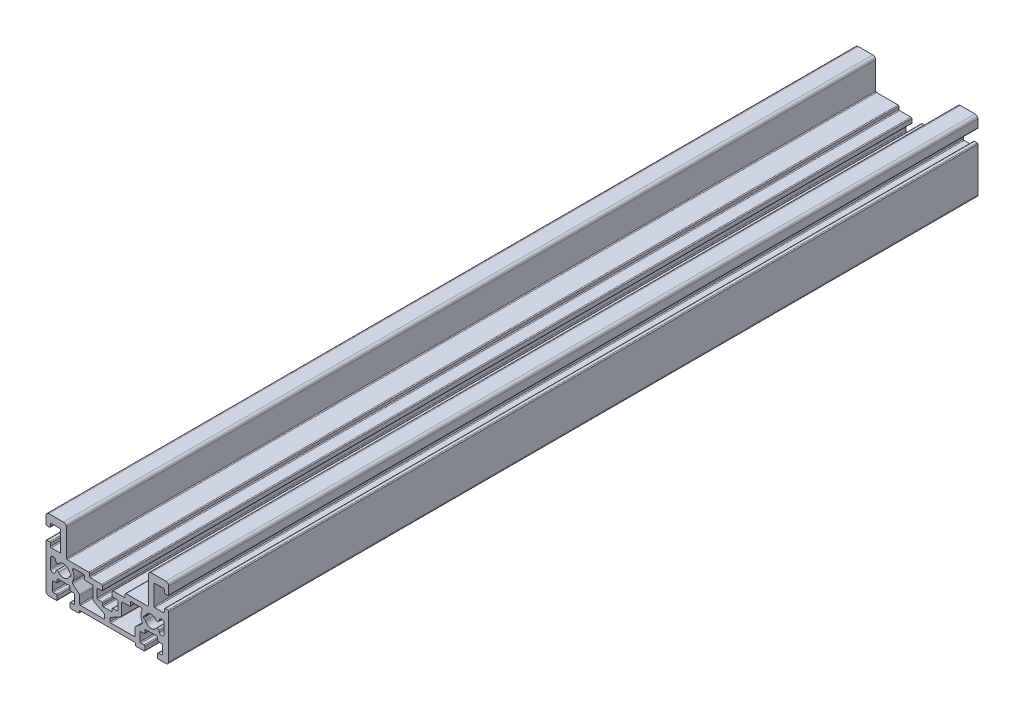
SolidWorks part; units mm, degrees
ref_plane "Front Plane" through (0, 0, 0) normal (0, 0, 1) x (1, 0, 0)
ref_plane "Top Plane" through (0, 0, 0) normal (0, 1, 0) x (1, 0, 0)
ref_plane "Right Plane" through (0, 0, 0) normal (1, 0, 0) x (0, 0, -1)
sketch "Sketch3" plane through (0, 0, 0) normal (0, 0, 1) x (1, 0, 0)
  line L214 (780.7533, -9071.888) -> (783.9435, -9071.888)
  line L215 (784.2435, -9072.188) -> (784.2435, -9073.188)
  line L216 (784.5435, -9073.488) -> (786.9435, -9073.488)
  line L217 (787.2435, -9073.788) -> (787.2435, -9077.8106)
  line L218 (787.399, -9078.0735) -> (791.0881, -9080.1025)
  line L219 (791.2435, -9080.3654) -> (791.2435, -9081.388)
  line L220 (790.9435, -9081.688) -> (782.9935, -9081.688)
  line L221 (782.6935, -9081.388) -> (782.6935, -9078.9167)
  line L222 (782.5205, -9078.5385) -> (780.2888, -9076.609)
  line L223 (772.6935, -9075.8786) -> (772.6935, -9072.6975)
  line L224 (779.4063, -9073.788) -> (779.3935, -9073.788)
  line L225 (779.6935, -9074.088) -> (779.6935, -9074.488)
  line L226 (779.3935, -9074.788) -> (779.4063, -9074.788)
  line L227 (803.9983, -9076.609) -> (801.7665, -9078.5385)
  line L228 (801.5935, -9078.9167) -> (801.5935, -9081.388)
  line L229 (801.2935, -9081.688) -> (793.3435, -9081.688)
  line L230 (793.0435, -9081.388) -> (793.0435, -9080.3654)
  line L231 (793.199, -9080.1025) -> (796.8881, -9078.0735)
  line L232 (797.0435, -9077.8106) -> (797.0435, -9073.788)
  line L233 (797.3435, -9073.488) -> (799.7435, -9073.488)
  line L234 (800.0435, -9073.188) -> (800.0435, -9072.188)
  line L235 (800.3435, -9071.888) -> (803.5338, -9071.888)
  line L236 (804.8808, -9074.788) -> (804.8935, -9074.788)
  line L237 (804.5935, -9074.488) -> (804.5935, -9074.088)
  line L238 (804.8935, -9073.788) -> (804.8808, -9073.788)
  line L239 (811.5935, -9072.6975) -> (811.5935, -9075.8786)
  line L240 (773.3435, -9082.188) -> (773.3435, -9079.388)
  line L241 (773.6435, -9079.088) -> (774.6935, -9079.088)
  line L242 (774.9935, -9078.788) -> (774.9935, -9077.988)
  line L243 (775.2935, -9077.688) -> (778.9935, -9077.688)
  line L244 (779.2935, -9077.988) -> (779.2935, -9078.788)
  line L245 (779.5935, -9079.088) -> (780.6435, -9079.088)
  line L246 (780.9435, -9079.388) -> (780.9435, -9082.188)
  line L247 (780.6435, -9082.488) -> (779.5935, -9082.488)
  line L248 (779.2935, -9082.788) -> (779.2935, -9083.988)
  line L249 (779.5935, -9084.288) -> (782.2435, -9084.288)
  line L250 (782.5435, -9083.988) -> (782.5435, -9083.588)
  line L251 (782.8435, -9083.288) -> (801.4435, -9083.288)
  line L252 (801.7435, -9083.588) -> (801.7435, -9083.988)
  line L253 (802.0435, -9084.288) -> (804.6935, -9084.288)
  line L254 (804.9935, -9083.988) -> (804.9935, -9082.788)
  line L255 (804.6935, -9082.488) -> (803.6435, -9082.488)
  line L256 (803.3435, -9082.188) -> (803.3435, -9079.388)
  line L257 (803.6435, -9079.088) -> (804.6935, -9079.088)
  line L258 (804.9935, -9078.788) -> (804.9935, -9077.988)
  line L259 (805.2935, -9077.688) -> (808.9935, -9077.688)
  line L260 (809.2935, -9077.988) -> (809.2935, -9078.788)
  line L261 (809.5935, -9079.088) -> (810.6435, -9079.088)
  line L262 (810.9435, -9079.388) -> (810.9435, -9082.188)
  line L263 (810.6435, -9082.488) -> (809.5935, -9082.488)
  line L264 (809.2935, -9082.788) -> (809.2935, -9083.988)
  line L265 (809.5935, -9084.288) -> (812.1435, -9084.288)
  line L266 (813.1435, -9083.288) -> (813.1435, -9068.388)
  line L267 (812.8435, -9068.088) -> (811.9435, -9068.088)
  line L268 (811.6435, -9068.388) -> (811.6435, -9069.288)
  line L269 (811.3435, -9069.588) -> (808.4435, -9069.588)
  line L270 (808.1435, -9069.288) -> (808.1435, -9062.688)
  line L271 (808.4435, -9062.388) -> (811.3435, -9062.388)
  line L272 (811.6435, -9062.688) -> (811.6435, -9063.488)
  line L273 (811.9435, -9063.788) -> (812.8435, -9063.788)
  line L274 (813.1435, -9063.488) -> (813.1435, -9060.888)
  line L275 (812.1435, -9059.888) -> (807.1435, -9059.888)
  line L276 (806.1435, -9060.888) -> (806.1435, -9070.088)
  line L277 (805.8435, -9070.388) -> (798.5435, -9070.388)
  line L278 (798.2435, -9070.688) -> (798.2435, -9071.488)
  line L279 (797.9435, -9071.788) -> (794.0935, -9071.788)
  line L280 (793.7935, -9072.088) -> (793.7935, -9073.388)
  line L281 (794.0935, -9073.688) -> (795.4435, -9073.688)
  line L282 (795.7435, -9073.988) -> (795.7435, -9076.688)
  line L283 (795.4435, -9076.988) -> (794.0935, -9076.988)
  line L284 (793.7935, -9077.288) -> (793.7935, -9077.888)
  line L285 (793.4935, -9078.188) -> (790.7935, -9078.188)
  line L286 (790.4935, -9077.888) -> (790.4935, -9077.288)
  line L287 (790.1935, -9076.988) -> (788.8435, -9076.988)
  line L288 (788.5435, -9076.688) -> (788.5435, -9073.988)
  line L289 (788.8435, -9073.688) -> (790.1935, -9073.688)
  line L290 (790.4935, -9073.388) -> (790.4935, -9072.088)
  line L291 (790.1935, -9071.788) -> (786.3435, -9071.788)
  line L292 (786.0435, -9071.488) -> (786.0435, -9070.688)
  line L293 (785.7435, -9070.388) -> (778.4435, -9070.388)
  line L294 (778.1435, -9070.088) -> (778.1435, -9060.888)
  line L295 (777.1435, -9059.888) -> (772.1435, -9059.888)
  line L296 (771.1435, -9060.888) -> (771.1435, -9063.488)
  line L297 (771.4435, -9063.788) -> (772.3435, -9063.788)
  line L298 (772.6435, -9063.488) -> (772.6435, -9062.688)
  line L299 (772.9435, -9062.388) -> (775.8435, -9062.388)
  line L300 (776.1435, -9062.688) -> (776.1435, -9069.288)
  line L301 (775.8435, -9069.588) -> (772.9435, -9069.588)
  line L302 (772.6435, -9069.288) -> (772.6435, -9068.388)
  line L303 (772.3435, -9068.088) -> (771.4435, -9068.088)
  line L304 (771.1435, -9068.388) -> (771.1435, -9083.288)
  line L305 (772.1435, -9084.288) -> (774.6935, -9084.288)
  line L306 (774.9935, -9083.988) -> (774.9935, -9082.788)
  line L307 (774.6935, -9082.488) -> (773.6435, -9082.488)
  arc A179 (780.7533, -9071.888) -> (780.3097, -9072.6188) centre (780.7533, -9072.388) ccw
  arc A180 (784.2435, -9072.188) -> (783.9435, -9071.888) centre (783.9435, -9072.188) ccw
  arc A181 (784.2435, -9073.188) -> (784.5435, -9073.488) centre (784.5435, -9073.188) ccw
  arc A182 (787.2435, -9073.788) -> (786.9435, -9073.488) centre (786.9435, -9073.788) ccw
  arc A183 (787.2435, -9077.8106) -> (787.399, -9078.0735) centre (787.5435, -9077.8106) ccw
  arc A184 (791.2435, -9080.3654) -> (791.0881, -9080.1025) centre (790.9435, -9080.3654) ccw
  arc A185 (790.9435, -9081.688) -> (791.2435, -9081.388) centre (790.9435, -9081.388) ccw
  arc A186 (782.6935, -9081.388) -> (782.9935, -9081.688) centre (782.9935, -9081.388) ccw
  arc A187 (782.6935, -9078.9167) -> (782.5205, -9078.5385) centre (782.1935, -9078.9167) ccw
  arc A188 (780.1898, -9075.9689) -> (780.2888, -9076.609) centre (780.6158, -9076.2308) ccw
  arc A189 (780.1898, -9075.9689) -> (780.3097, -9072.6188) centre (777.2935, -9074.188) ccw
  arc A190 (779.4063, -9074.788) -> (779.1234, -9074.988) centre (779.4063, -9075.088) ccw
  arc A191 (775.4314, -9075.504) -> (779.1234, -9074.988) centre (777.1435, -9074.288) ccw
  arc A192 (775.4314, -9075.504) -> (774.5166, -9075.672) centre (775.0131, -9075.8011) ccw
  arc A193 (774.3604, -9076.1731) -> (774.5166, -9075.672) centre (769.1935, -9074.288) ccw
  arc A194 (772.6935, -9075.8786) -> (774.3604, -9076.1731) centre (773.553, -9075.8786) ccw
  arc A195 (774.3604, -9072.4029) -> (772.6935, -9072.6975) centre (773.553, -9072.6975) ccw
  arc A196 (774.5166, -9072.9041) -> (774.3604, -9072.4029) centre (769.1935, -9074.288) ccw
  arc A197 (774.5166, -9072.9041) -> (775.4314, -9073.072) centre (775.0131, -9072.775) ccw
  arc A198 (779.1234, -9073.588) -> (775.4314, -9073.072) centre (777.1435, -9074.288) ccw
  arc A199 (779.1234, -9073.588) -> (779.4063, -9073.788) centre (779.4063, -9073.488) ccw
  arc A200 (779.6935, -9074.088) -> (779.3935, -9073.788) centre (779.3935, -9074.088) ccw
  arc A201 (779.3935, -9074.788) -> (779.6935, -9074.488) centre (779.3935, -9074.488) ccw
  arc A202 (803.9773, -9072.6188) -> (803.5338, -9071.888) centre (803.5338, -9072.388) ccw
  arc A203 (803.9773, -9072.6188) -> (804.0972, -9075.9689) centre (806.9935, -9074.188) ccw
  arc A204 (803.9983, -9076.609) -> (804.0972, -9075.9689) centre (803.6713, -9076.2308) ccw
  arc A205 (801.7665, -9078.5385) -> (801.5935, -9078.9167) centre (802.0935, -9078.9167) ccw
  arc A206 (801.2935, -9081.688) -> (801.5935, -9081.388) centre (801.2935, -9081.388) ccw
  arc A207 (793.0435, -9081.388) -> (793.3435, -9081.688) centre (793.3435, -9081.388) ccw
  arc A208 (793.199, -9080.1025) -> (793.0435, -9080.3654) centre (793.3435, -9080.3654) ccw
  arc A209 (796.8881, -9078.0735) -> (797.0435, -9077.8106) centre (796.7435, -9077.8106) ccw
  arc A210 (797.3435, -9073.488) -> (797.0435, -9073.788) centre (797.3435, -9073.788) ccw
  arc A211 (799.7435, -9073.488) -> (800.0435, -9073.188) centre (799.7435, -9073.188) ccw
  arc A212 (800.3435, -9071.888) -> (800.0435, -9072.188) centre (800.3435, -9072.188) ccw
  arc A213 (805.1636, -9074.988) -> (804.8808, -9074.788) centre (804.8808, -9075.088) ccw
  arc A214 (804.5935, -9074.488) -> (804.8935, -9074.788) centre (804.8935, -9074.488) ccw
  arc A215 (804.8935, -9073.788) -> (804.5935, -9074.088) centre (804.8935, -9074.088) ccw
  arc A216 (804.8808, -9073.788) -> (805.1636, -9073.588) centre (804.8808, -9073.488) ccw
  arc A217 (808.8557, -9073.072) -> (805.1636, -9073.588) centre (807.1435, -9074.288) ccw
  arc A218 (808.8557, -9073.072) -> (809.7705, -9072.9041) centre (809.274, -9072.775) ccw
  arc A219 (809.9267, -9072.4029) -> (809.7705, -9072.9041) centre (815.0935, -9074.288) ccw
  arc A220 (811.5935, -9072.6975) -> (809.9267, -9072.4029) centre (810.7341, -9072.6975) ccw
  arc A221 (809.9267, -9076.1731) -> (811.5935, -9075.8786) centre (810.7341, -9075.8786) ccw
  arc A222 (809.7705, -9075.672) -> (809.9267, -9076.1731) centre (815.0935, -9074.288) ccw
  arc A223 (809.7705, -9075.672) -> (808.8557, -9075.504) centre (809.274, -9075.8011) ccw
  arc A224 (805.1636, -9074.988) -> (808.8557, -9075.504) centre (807.1435, -9074.288) ccw
  arc A225 (773.6435, -9079.088) -> (773.3435, -9079.388) centre (773.6435, -9079.388) ccw
  arc A226 (774.6935, -9079.088) -> (774.9935, -9078.788) centre (774.6935, -9078.788) ccw
  arc A227 (775.2935, -9077.688) -> (774.9935, -9077.988) centre (775.2935, -9077.988) ccw
  arc A228 (779.2935, -9077.988) -> (778.9935, -9077.688) centre (778.9935, -9077.988) ccw
  arc A229 (779.2935, -9078.788) -> (779.5935, -9079.088) centre (779.5935, -9078.788) ccw
  arc A230 (780.9435, -9079.388) -> (780.6435, -9079.088) centre (780.6435, -9079.388) ccw
  arc A231 (780.6435, -9082.488) -> (780.9435, -9082.188) centre (780.6435, -9082.188) ccw
  arc A232 (779.5935, -9082.488) -> (779.2935, -9082.788) centre (779.5935, -9082.788) ccw
  arc A233 (779.2935, -9083.988) -> (779.5935, -9084.288) centre (779.5935, -9083.988) ccw
  arc A234 (782.2435, -9084.288) -> (782.5435, -9083.988) centre (782.2435, -9083.988) ccw
  arc A235 (782.8435, -9083.288) -> (782.5435, -9083.588) centre (782.8435, -9083.588) ccw
  arc A236 (801.7435, -9083.588) -> (801.4435, -9083.288) centre (801.4435, -9083.588) ccw
  arc A237 (801.7435, -9083.988) -> (802.0435, -9084.288) centre (802.0435, -9083.988) ccw
  arc A238 (804.6935, -9084.288) -> (804.9935, -9083.988) centre (804.6935, -9083.988) ccw
  arc A239 (804.9935, -9082.788) -> (804.6935, -9082.488) centre (804.6935, -9082.788) ccw
  arc A240 (803.3435, -9082.188) -> (803.6435, -9082.488) centre (803.6435, -9082.188) ccw
  arc A241 (803.6435, -9079.088) -> (803.3435, -9079.388) centre (803.6435, -9079.388) ccw
  arc A242 (804.6935, -9079.088) -> (804.9935, -9078.788) centre (804.6935, -9078.788) ccw
  arc A243 (805.2935, -9077.688) -> (804.9935, -9077.988) centre (805.2935, -9077.988) ccw
  arc A244 (809.2935, -9077.988) -> (808.9935, -9077.688) centre (808.9935, -9077.988) ccw
  arc A245 (809.2935, -9078.788) -> (809.5935, -9079.088) centre (809.5935, -9078.788) ccw
  arc A246 (810.9435, -9079.388) -> (810.6435, -9079.088) centre (810.6435, -9079.388) ccw
  arc A247 (810.6435, -9082.488) -> (810.9435, -9082.188) centre (810.6435, -9082.188) ccw
  arc A248 (809.5935, -9082.488) -> (809.2935, -9082.788) centre (809.5935, -9082.788) ccw
  arc A249 (809.2935, -9083.988) -> (809.5935, -9084.288) centre (809.5935, -9083.988) ccw
  arc A250 (812.1435, -9084.288) -> (813.1435, -9083.288) centre (812.1435, -9083.288) ccw
  arc A251 (813.1435, -9068.388) -> (812.8435, -9068.088) centre (812.8435, -9068.388) ccw
  arc A252 (811.9435, -9068.088) -> (811.6435, -9068.388) centre (811.9435, -9068.388) ccw
  arc A253 (811.3435, -9069.588) -> (811.6435, -9069.288) centre (811.3435, -9069.288) ccw
  arc A254 (808.1435, -9069.288) -> (808.4435, -9069.588) centre (808.4435, -9069.288) ccw
  arc A255 (808.4435, -9062.388) -> (808.1435, -9062.688) centre (808.4435, -9062.688) ccw
  arc A256 (811.6435, -9062.688) -> (811.3435, -9062.388) centre (811.3435, -9062.688) ccw
  arc A257 (811.6435, -9063.488) -> (811.9435, -9063.788) centre (811.9435, -9063.488) ccw
  arc A258 (812.8435, -9063.788) -> (813.1435, -9063.488) centre (812.8435, -9063.488) ccw
  arc A259 (813.1435, -9060.888) -> (812.1435, -9059.888) centre (812.1435, -9060.888) ccw
  arc A260 (807.1435, -9059.888) -> (806.1435, -9060.888) centre (807.1435, -9060.888) ccw
  arc A261 (805.8435, -9070.388) -> (806.1435, -9070.088) centre (805.8435, -9070.088) ccw
  arc A262 (798.5435, -9070.388) -> (798.2435, -9070.688) centre (798.5435, -9070.688) ccw
  arc A263 (797.9435, -9071.788) -> (798.2435, -9071.488) centre (797.9435, -9071.488) ccw
  arc A264 (794.0935, -9071.788) -> (793.7935, -9072.088) centre (794.0935, -9072.088) ccw
  arc A265 (793.7935, -9073.388) -> (794.0935, -9073.688) centre (794.0935, -9073.388) ccw
  arc A266 (795.7435, -9073.988) -> (795.4435, -9073.688) centre (795.4435, -9073.988) ccw
  arc A267 (795.4435, -9076.988) -> (795.7435, -9076.688) centre (795.4435, -9076.688) ccw
  arc A268 (794.0935, -9076.988) -> (793.7935, -9077.288) centre (794.0935, -9077.288) ccw
  arc A269 (793.4935, -9078.188) -> (793.7935, -9077.888) centre (793.4935, -9077.888) ccw
  arc A270 (790.4935, -9077.888) -> (790.7935, -9078.188) centre (790.7935, -9077.888) ccw
  arc A271 (790.4935, -9077.288) -> (790.1935, -9076.988) centre (790.1935, -9077.288) ccw
  arc A272 (788.5435, -9076.688) -> (788.8435, -9076.988) centre (788.8435, -9076.688) ccw
  arc A273 (788.8435, -9073.688) -> (788.5435, -9073.988) centre (788.8435, -9073.988) ccw
  arc A274 (790.1935, -9073.688) -> (790.4935, -9073.388) centre (790.1935, -9073.388) ccw
  arc A275 (790.4935, -9072.088) -> (790.1935, -9071.788) centre (790.1935, -9072.088) ccw
  arc A276 (786.0435, -9071.488) -> (786.3435, -9071.788) centre (786.3435, -9071.488) ccw
  arc A277 (786.0435, -9070.688) -> (785.7435, -9070.388) centre (785.7435, -9070.688) ccw
  arc A278 (778.1435, -9070.088) -> (778.4435, -9070.388) centre (778.4435, -9070.088) ccw
  arc A279 (778.1435, -9060.888) -> (777.1435, -9059.888) centre (777.1435, -9060.888) ccw
  arc A280 (772.1435, -9059.888) -> (771.1435, -9060.888) centre (772.1435, -9060.888) ccw
  arc A281 (771.1435, -9063.488) -> (771.4435, -9063.788) centre (771.4435, -9063.488) ccw
  arc A282 (772.3435, -9063.788) -> (772.6435, -9063.488) centre (772.3435, -9063.488) ccw
  arc A283 (772.9435, -9062.388) -> (772.6435, -9062.688) centre (772.9435, -9062.688) ccw
  arc A284 (776.1435, -9062.688) -> (775.8435, -9062.388) centre (775.8435, -9062.688) ccw
  arc A285 (775.8435, -9069.588) -> (776.1435, -9069.288) centre (775.8435, -9069.288) ccw
  arc A286 (772.6435, -9069.288) -> (772.9435, -9069.588) centre (772.9435, -9069.288) ccw
  arc A287 (772.6435, -9068.388) -> (772.3435, -9068.088) centre (772.3435, -9068.388) ccw
  arc A288 (771.4435, -9068.088) -> (771.1435, -9068.388) centre (771.4435, -9068.388) ccw
  arc A289 (771.1435, -9083.288) -> (772.1435, -9084.288) centre (772.1435, -9083.288) ccw
  arc A290 (774.6935, -9084.288) -> (774.9935, -9083.988) centre (774.6935, -9083.988) ccw
  arc A291 (774.9935, -9082.788) -> (774.6935, -9082.488) centre (774.6935, -9082.788) ccw
  arc A292 (773.3435, -9082.188) -> (773.6435, -9082.488) centre (773.6435, -9082.188) ccw
extrude "Boss-Extrude1" add sketch "Sketch3" along normal blind 147 and the other way blind 130
